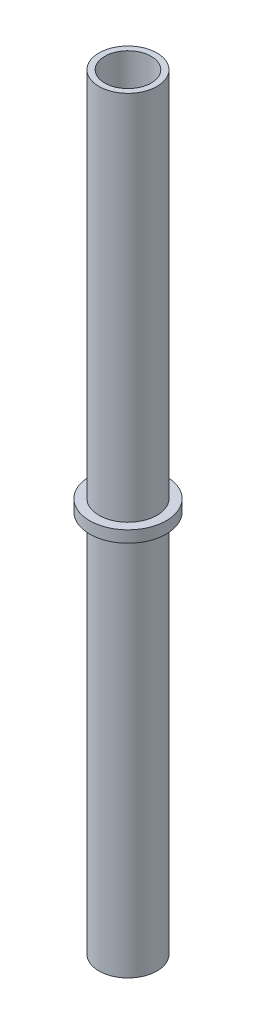
SolidWorks part; units mm, degrees
ref_plane "Front Plane" through (0, 0, 0) normal (0, 0, 1) x (1, 0, 0)
ref_plane "Top Plane" through (0, 0, 0) normal (0, 1, 0) x (1, 0, 0)
ref_plane "Right Plane" through (0, 0, 0) normal (1, 0, 0) x (0, 0, -1)
sketch "Sketch1" plane through (0, 0, 0) normal (0, 0, 1) x (1, 0, 0)
  line L0 (0, 0) -> (25, 0)
  line L1 (25, 0) -> (25, 330)
  line L2 (25, 330) -> (33, 330)
  line L3 (33, 330) -> (33, 340)
  line L4 (33, 340) -> (25, 340)
  line L5 (25, 340) -> (25, 585.1197)
  line L9 (25, 585.1197) -> (25, 619.0324)
  line L13 (25, 619.0324) -> (25, 660)
  line L14 (25, 660) -> (0, 660)
  line L15 (0, 660) -> (0, 0)
  dimension "D1" = 25
  dimension "D2" = 25
  dimension "D3" = 25
  dimension "D5" = 340
  dimension "D6" = 8
  dimension "D7" = 10
  dimension "D10" = 660
revolve "Revolve1" add sketch "Sketch1" angle 360 about L15
sketch "Sketch2" plane through (0, 660, 0) normal (0, 1, 0) x (1, 0, 0)
  circle A0 centre (0, 0) radius 20
extrude "Cut-Extrude1" cut sketch "Sketch2" against normal through all
